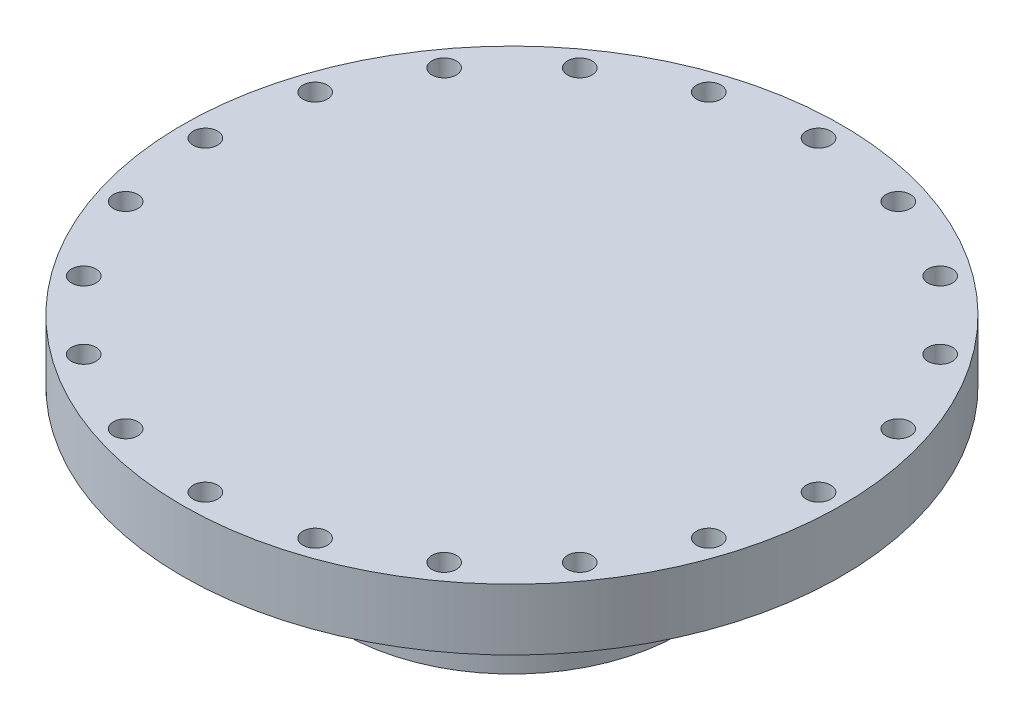
SolidWorks part; units mm, degrees
material "Q235B"
ref_plane "Front Plane" through (0, 0, 0) normal (0, 0, 1) x (1, 0, 0)
ref_plane "Top Plane" through (0, 0, 0) normal (0, 1, 0) x (1, 0, 0)
ref_plane "Right Plane" through (0, 0, 0) normal (1, 0, 0) x (0, 0, -1)
sketch "Sketch1" plane through (0, 0, 0) normal (0, 1, 0) x (1, 0, 0)
  line L1 (215, -400) -> (-215, -400)
  line L2 (215, -400) -> (215, 400)
  line L3 (215, 400) -> (-215, 400)
  line L4 (-215, -400) -> (-215, 400)
  line L5 (215, -400) -> (-215, 400) construction
  line L6 (215, 400) -> (-215, -400) construction
  circle A0 centre (0, 0) radius 215
  circle A1 centre (0, 0) radius 160
  dimension "D1" = 430
  dimension "D4" = 320
  dimension "D2" = 800
  dimension "D3" = 430
extrude "Boss-Extrude1" add sketch "Sketch1" along normal blind 40 contours L2 A0 L4 A1 | A1
hole_wizard "Ø16.0 (16) Diameter Hole1" positions "Sketch3" profile "Sketch4" hole size "Ø16.0" standard "GB" end condition up to next
sketch "Sketch3" plane through (0, 40, 0) normal (0, 1, 0) x (1, 0, 0)
  circle A0 centre (0, 0) radius 200 construction
  point P0 (200, 0)
  point P14 (190.2113, -61.8034)
  point P15 (161.8034, -117.5571)
  point P16 (117.5571, -161.8034)
  point P17 (61.8034, -190.2113)
  point P18 (0, -200)
  point P19 (-61.8034, -190.2113)
  point P20 (-117.5571, -161.8034)
  point P21 (-161.8034, -117.5571)
  point P22 (-190.2113, -61.8034)
  point P23 (-200, 0)
  point P24 (-190.2113, 61.8034)
  point P25 (-161.8034, 117.5571)
  point P26 (-117.5571, 161.8034)
  point P27 (-61.8034, 190.2113)
  point P28 (0, 200)
  point P29 (61.8034, 190.2113)
  point P30 (117.5571, 161.8034)
  point P31 (161.8034, 117.5571)
  point P32 (190.2113, 61.8034)
  dimension "D1" = 400
  dimension "D2" = 20
sketch "Sketch4" plane through (200, 40, 0) normal (1, 0, 0) x (0, 0, 1)
  line L0 (0, 0) -> (0, 40)
  line L1 (0, 40) -> (8, 40)
  line L2 (8, 40) -> (8, 0)
  line L5 (8, 0) -> (0, 0)
  line L11 (0, -6.35) -> (0, 107.95) construction
  dimension "通孔孔直径" = 16
  dimension "通孔孔深度" = 40
hole_wizard "G1/2 Tapped Hole1" positions "Sketch5" profile "Sketch6" tap size "G1/2" standard "GB"
sketch "Sketch5" plane through (0, 40, 0) normal (0, 1, 0) x (1, 0, 0)
  line L0 (0, 50.1035) -> (0, 0) construction
  line L1 (0, 0) -> (-60, 0) construction
  point P0 (-60, 0)
  point P8 (60, 0)
  dimension "D1" = 120
sketch "Sketch6" plane through (-60, 40, 0) normal (1, 0, 0) x (0, 0, 1)
  line L0 (0, 0) -> (0, 40)
  line L1 (0, 40) -> (9.5, 40)
  line L2 (9.5, 40) -> (9.5, 0)
  line L5 (9.5, 0) -> (0, 0)
  line L11 (0, -6.35) -> (0, 107.95) construction
  dimension "通孔螺纹孔钻头直径" = 19
  dimension "通孔螺纹孔钻头深度" = 40
cosmetic thread "CosmeticThread1" [suppressed] parameters "D2"=20.955
cosmetic thread "CosmeticThread2" [suppressed] parameters "D2"=20.955
sketch "Sketch7" plane through (0, 0, 0) normal (0, -1, 0) x (1, 0, 0)
  circle A0 centre (0, 0) radius 110
  circle A1 centre (0, 0) radius 40
  dimension "D1" = 220
  dimension "D2" = 80
extrude "Boss-Extrude2" add sketch "Sketch7" along normal blind 85
